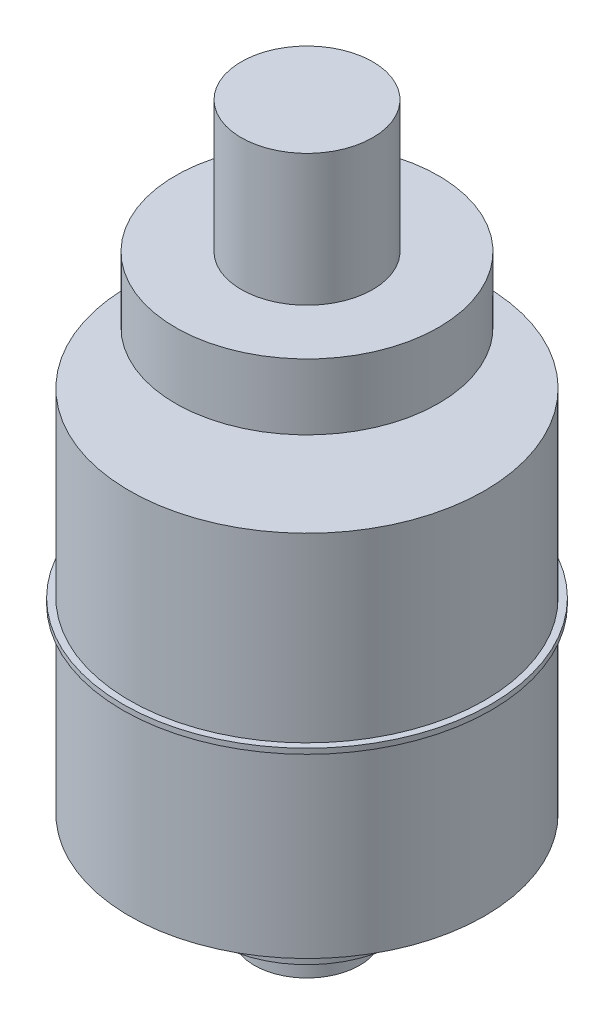
from build123d import *


with BuildPart() as part:
    # Sketch1 → Revolve1 (revolve)
    with BuildSketch(Plane.XY, mode=Mode.PRIVATE) as revolve1_sk:
        Polygon((0, 0), (0, 55), (-5, 55), (-5, 45), (-10, 45), (-10, 40), (-4, 40), (-4, 36), (-13.5, 36), (-13.5, 22.2), (-14, 22.2), (-14, 21.8), (-13.5, 21.8), (-13.5, 8), (-4, 8), (-4, 4), (-7, 4), (-7, 3), (-4, 3), (-4, 0), align=None)
    revolve(revolve1_sk.sketch.rotate(Axis((0, 0, 0), (0, 1, 0)), 180), axis=Axis((0, 0, 0), (0, 1, 0)))


solid = part.part
